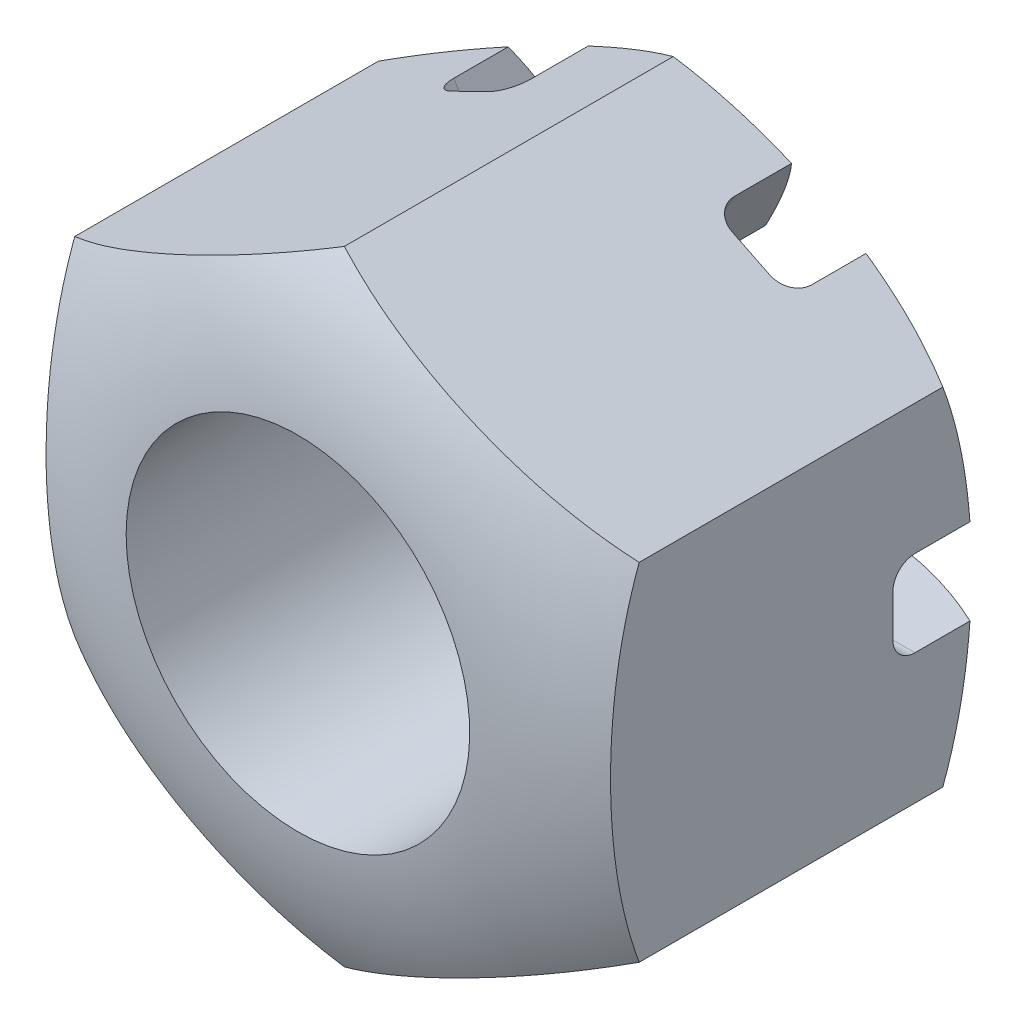
SolidWorks part; units mm, degrees
material "普通碳钢"
ref_plane "前视基准面" through (0, 0, 0) normal (0, 0, 1) x (1, 0, 0)
ref_plane "上视基准面" through (0, 0, 0) normal (0, 1, 0) x (1, 0, 0)
ref_plane "右视基准面" through (0, 0, 0) normal (1, 0, 0) x (0, 0, -1)
sketch "草图1" plane through (0, 0, 0) normal (0, 0, 1) x (1, 0, 0)
  line L0 (-103.5007, 0) -> (120.4894, 0) construction
  line L1 (0, 58.0231) -> (0, -56.7163) construction
  line L2 (0, 25.425) -> (-23.0001, 14.1137)
  line L3 (-23.0001, 14.1137) -> (-23.0001, -14.1137)
  line L6 (23.0001, -14.1137) -> (23.0001, 14.1137)
  line L7 (23.0001, 14.1137) -> (0, 25.425)
  line L8 (-23.0001, -14.1137) -> (0, -25.425)
  line L9 (0, -25.425) -> (23.0001, -14.1137)
  dimension "D1" = 46.0003
  dimension "D2" = 50.85
extrude "凸台-拉伸1" add sketch "草图1" along normal blind 34.6
sketch "草图3" plane through (0, 0, 0) normal (0, 0, -1) x (-1, 0, 0)
  line L0 (-32.5, 3.5) -> (32.5, 3.5)
  line L1 (32.5, 3.5) -> (32.5, -3.5)
  line L2 (-32.5, -3.5) -> (32.5, -3.5)
  line L3 (-32.5, -3.5) -> (-32.5, 3.5)
  line L4 (19.03, 0) -> (-19.03, 0) construction
  line L5 (0, 19.03) -> (0, -19.03) construction
  dimension "D1" = 65
  dimension "D2" = 3.5
  dimension "D3" = 7
  dimension "D4" = 32.5
extrude "切除-拉伸1" cut sketch "草图3" against normal blind 9
ref_axis "基准轴1" through (0, 0, -1.73) along (0, 0, 1)
pattern_circular "阵列(圆周)1" count 3 over 120 about axis through (0, 0, 0) along (0, 0, 1) of "切除-拉伸1"
hole_wizard "M30x2.0 螺纹孔1" positions "草图7" profile "草图6" tap size "M30x2.0" standard "GB" end condition through all
sketch "草图7" plane through (0, 0, 34.6) normal (0, 0, 1) x (1, 0, 0)
  point P0 (0, 0)
sketch "草图6" plane through (0, 0, 34.6) normal (1, 0, 0) x (0, -1, 0)
  line L0 (0, 0) -> (0, 34.6)
  line L1 (0, 34.6) -> (14, 34.6)
  line L2 (14, 34.6) -> (14, 0)
  line L5 (14, 0) -> (0, 0)
  line L11 (0, -6.35) -> (0, 107.95) construction
  dimension "通孔螺纹孔钻头直径" = 28
  dimension "通孔螺纹孔钻头深度" = 34.6
cosmetic thread "孔螺蚊线1" parameters "D2"=30
fillet "圆角2" radius 1.8 8 edges at (-12.1947, -14.1219, 9) (-6.0159, -17.4199, 9) (-12.1947, 14.1219, 9) (-6.0159, 17.4199, 9) (18.2778, -3.5, 9) (18.2778, 3.5, 9) (12.1947, 14.1219, 9) (6.0159, 17.4199, 9)
sketch "草图8" plane through (0, 0, 0) normal (0, 1, 0) x (1, 0, 0)
  line L0 (0, -19.03) -> (0, 19.03) construction
  line L1 (23.0001, 0) -> (14.5806, 0) construction
  line L2 (23.0001, -34.6) -> (0, -34.6) construction
  line L3 (11.5, 0) -> (33.5205, 0)
  line L4 (33.5205, 0) -> (33.5205, -11.5246)
  line L6 (11.5, -34.6) -> (33.5205, -34.6)
  line L7 (33.5205, -34.6) -> (33.5205, -23.0754)
  arc A0 (11.5, -34.6) -> (33.5205, -23.0754) centre (11.5, -7.8) ccw
  arc A1 (33.5205, -11.5246) -> (11.5, 0) centre (11.5, -26.8) ccw
  dimension "D1" = 53.6
  dimension "D4" = 11.5
  dimension "D6" = 53.6
  dimension "D2" = 11.5
  dimension "D3" = 26.8
  dimension "D5" = 26.8
revolve "切除-旋转1" cut sketch "草图8" angle 360 about axis through (0, 0, -1.73) along (0, 0, 1)
